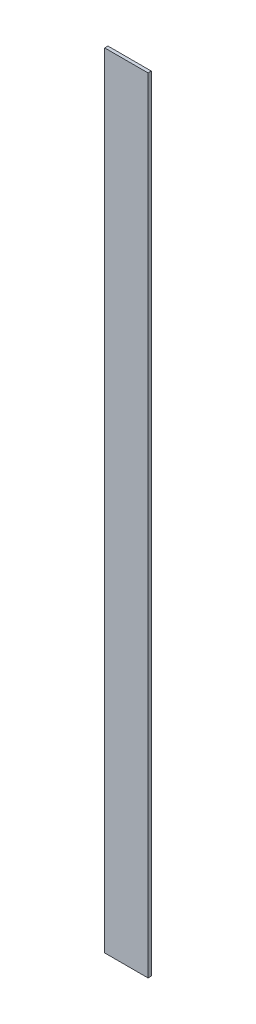
from build123d import *

# Parameters (mm, degrees)
SKETCH1_W           = 400
SKETCH1_H           = 7226
BOSS_EXTRUDE1_DEPTH = 15


with BuildPart() as part:
    # Sketch1 → Boss-Extrude1 (new, symmetric)
    with BuildSketch(Plane.XY):
        Rectangle(SKETCH1_W, SKETCH1_H)
    extrude(amount=BOSS_EXTRUDE1_DEPTH, both=True)


solid = part.part
